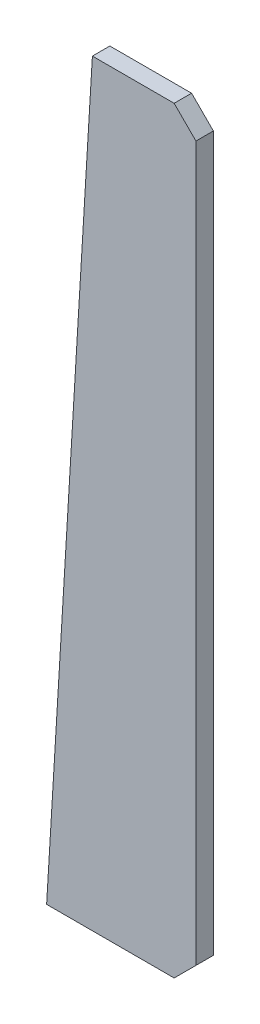
SolidWorks part; units mm, degrees
material "Q235B"
ref_plane "前视基准面" through (0, 0, 0) normal (0, 0, 1) x (1, 0, 0)
ref_plane "上视基准面" through (0, 0, 0) normal (0, 1, 0) x (1, 0, 0)
ref_plane "右视基准面" through (0, 0, 0) normal (1, 0, 0) x (0, 0, -1)
sketch "草图2" plane through (0, 0, 0) normal (0, 0, 1) x (1, 0, 0)
  line L0 (0, 0) -> (42, 695)
  line L1 (42, 695) -> (137, 695)
  line L2 (137, 695) -> (137, 0)
  line L3 (137, 0) -> (0, 0)
  dimension "D1" = 137
  dimension "D2" = 695
  dimension "D3" = 95
extrude "凸台-拉伸1" add sketch "草图2" along normal mid plane 16
chamfer "倒角1" distance 20 angle 45 2 edges at (137, 0, 0) (137, 695, 0)
